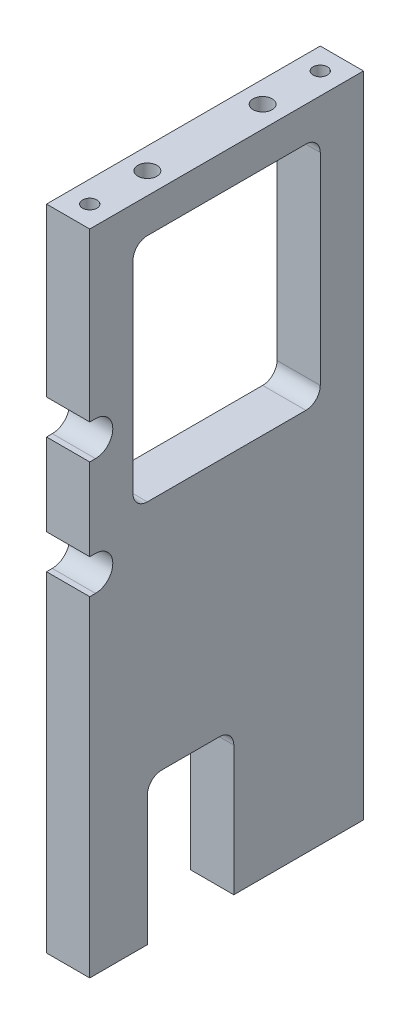
from build123d import *

# Parameters (mm, degrees)
SKETCH1_W                  = 95
SKETCH1_H                  = 225.1
BOSS_EXTRUDE1_DEPTH        = 15
CUT_EXTRUDE1_DEPTH         = 124.080268524
M6_CLEARANCE_HOLE1_D       = 6.6
M6_CLEARANCE_HOLE1_DEPTH   = 19.75
M6_CLEARANCE_HOLE1_TIP     = 1.982840043
M6_TAPPED_HOLE1_D          = 5
M6_TAPPED_HOLE1_DEPTH      = 15
M6_TAPPED_HOLE1_TIP        = 1.502151548
F_5_0MM_BLIND_HOLE_1_D     = 5
F_5_0MM_BLIND_HOLE_1_DEPTH = 8
F_5_0MM_BLIND_HOLE_1_TIP   = 1.502151548
F_5_0MM_BLIND_HOLE_2_D     = 5
F_5_0MM_BLIND_HOLE_2_DEPTH = 8
F_5_0MM_BLIND_HOLE_2_TIP   = 1.502151548
SKETCH14_R                 = 6
CUT_EXTRUDE2_DEPTH         = 124.080268524
SKETCH15_W                 = 10
SKETCH15_H                 = 12
CUT_EXTRUDE3_DEPTH         = 124.080268524
M5_TAPPED_HOLE1_AT_2_COUNT = 2
M5_TAPPED_HOLE1_AT_2_PITCH = 145


with BuildPart() as part:
    # Sketch1 → Boss-Extrude1 (new body)
    with BuildSketch(Plane(origin=(0, 0, 0), x_dir=(0, 0, -1), z_dir=(1, 0, 0))):
        Rectangle(SKETCH1_W, SKETCH1_H)
    extrude(amount=BOSS_EXTRUDE1_DEPTH)

    # Sketch2 → Cut-Extrude1 (cut, through all)
    with BuildSketch(Plane.ZY):
        with BuildLine():
            Line((22.5, -62.55), (2.5, -62.55))
            ThreePointArc((2.5, -62.55), (-1.035533906, -64.014466094), (-2.5, -67.55))
            Line((-2.5, -67.55), (-2.5, -112.55))
            Line((-2.5, -112.55), (27.5, -112.55))
            Line((27.5, -112.55), (27.5, -67.55))
            ThreePointArc((27.5, -67.55), (26.035533906, -64.014466094), (22.5, -62.55))
        make_face()
        with BuildLine():
            Line((-27.5, 20.55), (27.5, 20.55))
            ThreePointArc((27.5, 20.55), (31.035533906, 22.014466094), (32.5, 25.55))
            Line((32.5, 25.55), (32.5, 95.55))
            ThreePointArc((32.5, 95.55), (31.035533906, 99.085533906), (27.5, 100.55))
            Line((27.5, 100.55), (-27.5, 100.55))
            ThreePointArc((-27.5, 100.55), (-31.035533906, 99.085533906), (-32.5, 95.55))
            Line((-32.5, 95.55), (-32.5, 25.55))
            ThreePointArc((-32.5, 25.55), (-31.035533906, 22.014466094), (-27.5, 20.55))
        make_face()
    extrude(amount=-CUT_EXTRUDE1_DEPTH, mode=Mode.SUBTRACT)

    # M6 Clearance Hole1
    with Locations(Plane(origin=(0, 112.55, 0), x_dir=(1, 0, 0), z_dir=(0, 1, 0))):
        with Locations((7.5, -20), (7.5, 20)):
            Hole(M6_CLEARANCE_HOLE1_D / 2, depth=M6_CLEARANCE_HOLE1_DEPTH)
            with Locations((0, 0, -(M6_CLEARANCE_HOLE1_DEPTH + M6_CLEARANCE_HOLE1_TIP / 2))):  # 118° drill point
                Cone(0, M6_CLEARANCE_HOLE1_D / 2, M6_CLEARANCE_HOLE1_TIP, mode=Mode.SUBTRACT)

    # M6 Tapped Hole1
    with Locations(Plane(origin=(0, -112.55, 0), x_dir=(-1, 0, 0), z_dir=(0, -1, 0))):
        with Locations((-7.5, -40), (-7.5, 40)):
            Hole(M6_TAPPED_HOLE1_D / 2, depth=M6_TAPPED_HOLE1_DEPTH)
            with Locations((0, 0, -(M6_TAPPED_HOLE1_DEPTH + M6_TAPPED_HOLE1_TIP / 2))):  # 118° drill point
                Cone(0, M6_TAPPED_HOLE1_D / 2, M6_TAPPED_HOLE1_TIP, mode=Mode.SUBTRACT)

    # Ø5.0mm blind hole 1
    with Locations(Plane(origin=(0, -112.55, 0), x_dir=(-1, 0, 0), z_dir=(0, -1, 0))):
        with Locations((-7.5, 10)):
            Hole(F_5_0MM_BLIND_HOLE_1_D / 2, depth=F_5_0MM_BLIND_HOLE_1_DEPTH)
            with Locations((0, 0, -(F_5_0MM_BLIND_HOLE_1_DEPTH + F_5_0MM_BLIND_HOLE_1_TIP / 2))):  # 118° drill point
                Cone(0, F_5_0MM_BLIND_HOLE_1_D / 2, F_5_0MM_BLIND_HOLE_1_TIP, mode=Mode.SUBTRACT)

    # Ø5.0mm blind hole 2
    with Locations(Plane(origin=(0, 112.55, 0), x_dir=(1, 0, 0), z_dir=(0, 1, 0))):
        with Locations((7.5, -40), (7.5, 40)):
            Hole(F_5_0MM_BLIND_HOLE_2_D / 2, depth=F_5_0MM_BLIND_HOLE_2_DEPTH)
            with Locations((0, 0, -(F_5_0MM_BLIND_HOLE_2_DEPTH + F_5_0MM_BLIND_HOLE_2_TIP / 2))):  # 118° drill point
                Cone(0, F_5_0MM_BLIND_HOLE_2_D / 2, F_5_0MM_BLIND_HOLE_2_TIP, mode=Mode.SUBTRACT)

    # Sketch14 → Cut-Extrude2 (cut, through all)
    with BuildSketch(Plane(origin=(15, 0, 0), x_dir=(0, 0, -1), z_dir=(1, 0, 0))):
        with Locations((-45.5, 48.55)):
            Circle(SKETCH14_R)
        with Locations((-45.5, 8.05)):
            Circle(SKETCH14_R)
    extrude(amount=-CUT_EXTRUDE2_DEPTH, mode=Mode.SUBTRACT)

    # Sketch15 → Cut-Extrude3 (cut, through all)
    with BuildSketch(Plane.ZY):
        with Locations((50.5, 8.05)):
            Rectangle(SKETCH15_W, SKETCH15_H)
        with Locations((50.5, 48.55)):
            Rectangle(SKETCH15_W, SKETCH15_H)
    extrude(amount=-CUT_EXTRUDE3_DEPTH, mode=Mode.SUBTRACT)

    # Sketch19 → M5 Tapped Hole1 (revolve, cut)
    with BuildSketch(Plane(origin=(0, -77.45, -40), x_dir=(0, 0, 1), z_dir=(0, 1, 0))):
        Polygon((0, 0), (0, 13.6618073), (2.1, 12.4), (2.1, 0), align=None)
    m5_tapped_hole1 = revolve(axis=Axis((-6.35, -77.45, -40), (1, 0, 0)), mode=Mode.SUBTRACT)

    # M5 Tapped Hole1 at 2: M5 Tapped Hole1 ×2
    with Locations(*[(0, i * M5_TAPPED_HOLE1_AT_2_PITCH, 0) for i in range(1, M5_TAPPED_HOLE1_AT_2_COUNT)]):
        add(m5_tapped_hole1, mode=Mode.SUBTRACT)

    # Mirror1: M5 Tapped Hole1 across plane
    add(m5_tapped_hole1.mirror(Plane.XY), mode=Mode.SUBTRACT)

    # Mirror1 copy 1 sketch → Mirror1 copy 1 (revolve, cut)
    with BuildSketch(Plane(origin=(0, 67.55, 40), x_dir=(0, 0, -1), z_dir=(0, 1, 0))):
        Polygon((0, 0), (0, -13.6618073), (2.1, -12.4), (2.1, 0), align=None)
    revolve(axis=Axis((-6.35, 67.55, 40), (-1, 0, 0)), mode=Mode.SUBTRACT)


solid = part.part
